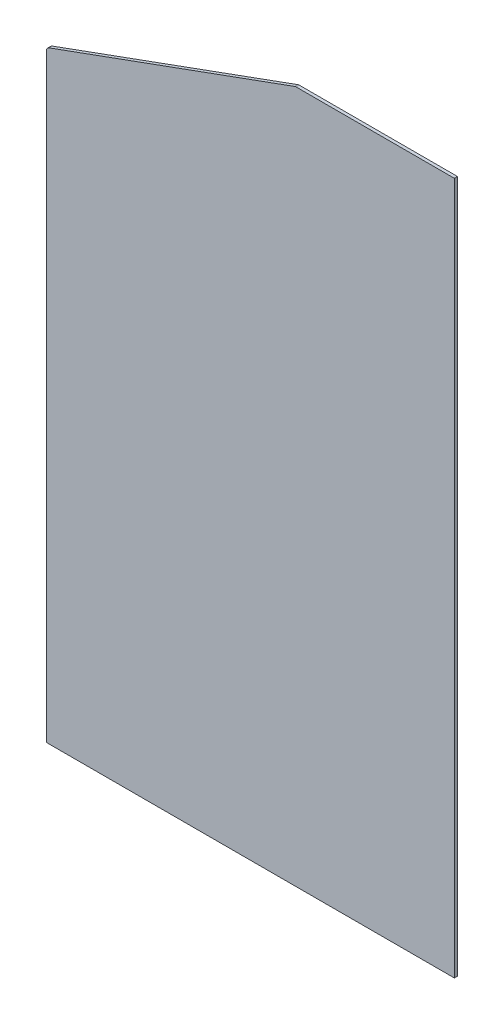
SolidWorks part; units mm, degrees
material "Q235B"
ref_plane "Front Plane" through (0, 0, 0) normal (0, 0, 1) x (1, 0, 0)
ref_plane "Top Plane" through (0, 0, 0) normal (0, 1, 0) x (1, 0, 0)
ref_plane "Right Plane" through (0, 0, 0) normal (1, 0, 0) x (0, 0, -1)
sketch "Sketch1" plane through (0, 0, 0) normal (0, 0, 1) x (1, 0, 0)
  line L0 (0, 0) -> (0, 1105.5)
  line L1 (0, 1105.5) -> (-253.62, 1105.5)
  line L2 (-253.62, 1105.5) -> (-651, 960.8655)
  line L3 (-651, 960.8655) -> (-651, 0)
  line L4 (-651, 0) -> (0, 0)
  dimension "D1" = 1105.5
  dimension "D2" = 253.62
  dimension "D3" = 160
  dimension "D4" = 651
extrude "Boss-Extrude1" add sketch "Sketch1" along normal blind 5
fillet "Fillet1" radius 6 2 edges at (-253.62, 1105.5, 2.5) (-651, 960.8655, 2.5)
